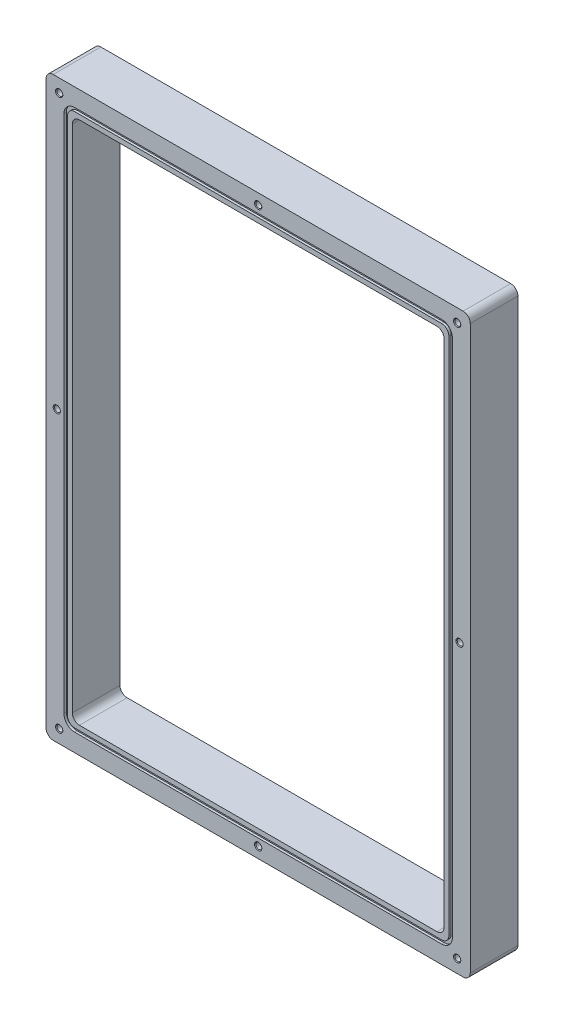
SolidWorks part; units mm, degrees
ref_plane "Front Plane" through (0, 0, 0) normal (0, 0, 1) x (1, 0, 0)
ref_plane "Top Plane" through (0, 0, 0) normal (0, 1, 0) x (1, 0, 0)
ref_plane "Right Plane" through (0, 0, 0) normal (1, 0, 0) x (0, 0, -1)
sketch "Sketch1" plane through (0, 0, 0) normal (0, 0, 1) x (1, 0, 0)
  line L0 (-89, 121) -> (-89, -121)
  line L1 (-78, 110) -> (78, 110)
  line L2 (-78, 110) -> (-78, -110)
  line L3 (-78, -110) -> (78, -110)
  line L4 (78, 110) -> (78, -110)
  line L5 (-78, 110) -> (78, -110) construction
  line L6 (-78, -110) -> (78, 110) construction
  line L7 (-89, -121) -> (89, -121)
  line L8 (89, 121) -> (89, -121)
  line L9 (-89, 121) -> (89, 121)
  point P0 (0, 0)
  dimension "D1" = 220
  dimension "D2" = 156
  dimension "D3" = 11
extrude "Boss-Extrude1" add sketch "Sketch1" along normal blind 20
fillet "Fillet1" radius 3 8 edges at (-89, 121, 10) (89, 121, 10) (89, -121, 10) (-89, -121, 10) (78, -110, 10) (-78, -110, 10) (78, 110, 10) (-78, 110, 10)
sketch "Sketch2" plane through (0, 0, 20) normal (0, 0, 1) x (1, 0, 0)
  line L0 (-81.5, 109) -> (-81.5, -109)
  line L1 (-77, -113.5) -> (77, -113.5)
  line L2 (81.5, -109) -> (81.5, 109)
  line L3 (77, 113.5) -> (-77, 113.5)
  line L23 (-75, -112) -> (75, -112)
  line L24 (80, -107) -> (80, 107)
  line L25 (-80, 107) -> (-80, -107)
  line L26 (75, 112) -> (-75, 112)
  line L27 (-77, -112) -> (77, -112)
  line L28 (80, -109) -> (80, 109)
  line L29 (-80, 109) -> (-80, -109)
  line L30 (77, 112) -> (-77, 112)
  arc A0 (-77, -112) -> (-80, -109) centre (-77, -109) cw
  arc A1 (77, -112) -> (80, -109) centre (77, -109) ccw
  arc A2 (77, 112) -> (80, 109) centre (77, 109) cw
  arc A3 (-77, 112) -> (-80, 109) centre (-77, 109) ccw
  arc A4 (-77, -113.5) -> (-81.5, -109) centre (-77, -109) cw
  arc A5 (77, -113.5) -> (81.5, -109) centre (77, -109) ccw
  arc A6 (77, 113.5) -> (81.5, 109) centre (77, 109) cw
  arc A7 (-77, 113.5) -> (-81.5, 109) centre (-77, 109) ccw
  arc A21 (-80, -107) -> (-75, -112) centre (-75, -107) ccw
  arc A22 (75, -112) -> (80, -107) centre (75, -107) ccw
  arc A23 (80, 107) -> (75, 112) centre (75, 107) ccw
  arc A24 (-75, 112) -> (-80, 107) centre (-75, 107) ccw
  dimension "D2" = 3
  dimension "D1" = 2
  dimension "D3" = 1.5
extrude "Cut-Extrude1" cut sketch "Sketch2" against normal blind 1
hole_wizard "M3 Tapped Hole2" positions "Sketch6" profile "Sketch7" tap size "M3" standard "GB"
sketch "Sketch6" plane through (0, 0, 20) normal (0, 0, 1) x (1, 0, 0)
  line L4 (-77, -113.5) -> (77, -113.5) construction
  line L5 (-81.5, 109) -> (-81.5, -109) construction
  line L6 (77, 113.5) -> (-77, 113.5) construction
  line L7 (81.5, -109) -> (81.5, 109) construction
  line L8 (77, 113.5) -> (-77, 113.5) construction
  point P0 (-83.5, 115.5)
  point P2 (0, 116.5)
  point P4 (83.5, 115.5)
  point P6 (-84.5, 0.0923)
  point P8 (84.5, -0.2344)
  point P10 (0, -116.5)
  point P12 (-83.5, -115.5)
  point P14 (83.5, -115.5)
  dimension "D1" = 3
  dimension "D2" = 3
  dimension "D3" = 3
  dimension "D4" = 3
  dimension "D5" = 2
  dimension "D6" = 2
  dimension "D7" = 2
  dimension "D8" = 2
sketch "Sketch7" plane through (-83.5, 115.5, 20) normal (1, 0, 0) x (0, -1, 0)
  line L0 (0, 0) -> (0, 7.2511)
  line L1 (0, 7.2511) -> (1.25, 6.5)
  line L2 (1.25, 6.5) -> (1.25, 0.275)
  line L3 (1.25, 0.275) -> (1.525, 0)
  line L5 (1.525, 0) -> (0, 0)
  line L6 (-1.25, 0.275) -> (-1.525, 0) construction
  line L10 (0, 7.2511) -> (-1.25, 6.5) construction
  line L11 (0, -6.35) -> (0, 107.95) construction
  dimension "螺纹孔钻头直径" = 2.5
  dimension "螺纹孔钻头深度" = 6.5
  dimension "近端锥形沉头孔直径" = 3.05
  dimension "近端锥形沉头孔角度" = 90
  dimension "导头角度" = 118
cosmetic thread "CosmeticThread thread 9" parameters "D1"=5, "D2"=3
cosmetic thread "CosmeticThread thread 10" parameters "D1"=5, "D2"=3
cosmetic thread "CosmeticThread thread 11" parameters "D1"=5, "D2"=3
cosmetic thread "CosmeticThread thread 12" parameters "D1"=5, "D2"=3
cosmetic thread "CosmeticThread thread 13" parameters "D1"=5, "D2"=3
cosmetic thread "CosmeticThread thread 14" parameters "D1"=5, "D2"=3
cosmetic thread "CosmeticThread thread 15" parameters "D1"=5, "D2"=3
cosmetic thread "CosmeticThread thread 16" parameters "D1"=5, "D2"=3
hole_wizard "M3 Tapped Hole1" positions "Sketch3" profile "Sketch4" tap size "M3" standard "GB"
sketch "Sketch3" plane through (0, 0, 0) normal (0, 0, -1) x (-1, 0, 0)
  line L0 (-75, 110) -> (75, 110) construction
  line L1 (-78, -107) -> (-78, 107) construction
  line L2 (78, 107) -> (78, -107) construction
  line L3 (75, -110) -> (-75, -110) construction
  point P0 (0, 113)
  point P2 (-81, 0)
  point P4 (81, 0)
  point P6 (0, -113)
  point P8 (80, -112)
  point P10 (-80, -112)
  point P12 (-80, 112)
  point P14 (80, 112)
  dimension "D1" = 3
  dimension "D2" = 3
  dimension "D3" = 3
  dimension "D4" = 3
  dimension "D5" = 2
  dimension "D6" = 2
  dimension "D7" = 2
  dimension "D8" = 2
  dimension "D9" = 2
  dimension "D10" = 2
  dimension "D11" = 2
  dimension "D12" = 2
sketch "Sketch4" plane through (0, 113, 0) normal (1, 0, 0) x (0, 1, 0)
  line L0 (0, 0) -> (0, 7.2511)
  line L1 (0, 7.2511) -> (1.25, 6.5)
  line L2 (1.25, 6.5) -> (1.25, 0.275)
  line L3 (1.25, 0.275) -> (1.525, 0)
  line L5 (1.525, 0) -> (0, 0)
  line L6 (-1.25, 0.275) -> (-1.525, 0) construction
  line L10 (0, 7.2511) -> (-1.25, 6.5) construction
  line L11 (0, -6.35) -> (0, 107.95) construction
  dimension "螺纹孔钻头直径" = 2.5
  dimension "螺纹孔钻头深度" = 6.5
  dimension "近端锥形沉头孔直径" = 3.05
  dimension "近端锥形沉头孔角度" = 90
  dimension "导头角度" = 118
cosmetic thread "CosmeticThread thread 1" parameters "D1"=5, "D2"=3
cosmetic thread "CosmeticThread thread 2" parameters "D1"=5, "D2"=3
cosmetic thread "CosmeticThread thread 3" parameters "D1"=5, "D2"=3
cosmetic thread "CosmeticThread thread 4" parameters "D1"=5, "D2"=3
cosmetic thread "CosmeticThread thread 5" parameters "D1"=5, "D2"=3
cosmetic thread "CosmeticThread thread 6" parameters "D1"=5, "D2"=3
cosmetic thread "CosmeticThread thread 7" parameters "D1"=5, "D2"=3
cosmetic thread "CosmeticThread thread 8" parameters "D1"=5, "D2"=3
sketch "Sketch5" plane through (0, 0, 0) normal (0, 0, -1) x (-1, 0, 0)
  line L38 (-84.5, 113.5) -> (-84.5, -113.5)
  line L39 (-81.5, -116.5) -> (81.5, -116.5)
  line L40 (84.5, -113.5) -> (84.5, 113.5)
  line L41 (81.5, 116.5) -> (-81.5, 116.5)
  line L42 (-86, -118) -> (86, -118)
  line L43 (86, -118) -> (86, 118)
  line L44 (86, 118) -> (-86, 118)
  line L45 (-86, 118) -> (-86, -118)
  line L46 (-81.5, -118) -> (81.5, -118)
  line L47 (86, -113.5) -> (86, 113.5)
  line L48 (81.5, 118) -> (-81.5, 118)
  line L49 (-86, 113.5) -> (-86, -113.5)
  line L50 (-84.5, 116.5) -> (-84.5, -116.5) construction
  line L51 (84.5, 116.5) -> (-84.5, 116.5) construction
  line L52 (84.5, -116.5) -> (84.5, 116.5) construction
  line L53 (-84.5, -116.5) -> (84.5, -116.5) construction
  line L54 (-86, -118) -> (86, -118) construction
  line L55 (-86, 118) -> (-86, -118) construction
  line L56 (86, -118) -> (86, 118) construction
  line L57 (86, 118) -> (-86, 118) construction
  arc A10 (-84.5, 113.5) -> (-81.5, 116.5) centre (-81.5, 113.5) cw
  arc A11 (84.5, 113.5) -> (81.5, 116.5) centre (81.5, 113.5) ccw
  arc A12 (81.5, -116.5) -> (84.5, -113.5) centre (81.5, -113.5) ccw
  arc A13 (-84.5, -113.5) -> (-81.5, -116.5) centre (-81.5, -113.5) ccw
  arc A22 (-81.5, -118) -> (-86, -113.5) centre (-81.5, -113.5) cw
  arc A23 (81.5, -118) -> (86, -113.5) centre (81.5, -113.5) ccw
  arc A24 (81.5, 118) -> (86, 113.5) centre (81.5, 113.5) cw
  arc A25 (-86, 113.5) -> (-81.5, 118) centre (-81.5, 113.5) cw
  dimension "D3" = 3
  dimension "D4" = 4.5
  dimension "D1" = 3
  dimension "D2" = 1.5
extrude "Cut-Extrude2" cut sketch "Sketch5" against normal blind 1
other "Move Face1" [suppressed] parameters "D1"=1.5
other "Move Face2" [suppressed] parameters "D1"=1.5
other "Move Face3" [suppressed] parameters "D1"=1.5
other "Move Face4" [suppressed] parameters "D1"=1.5
